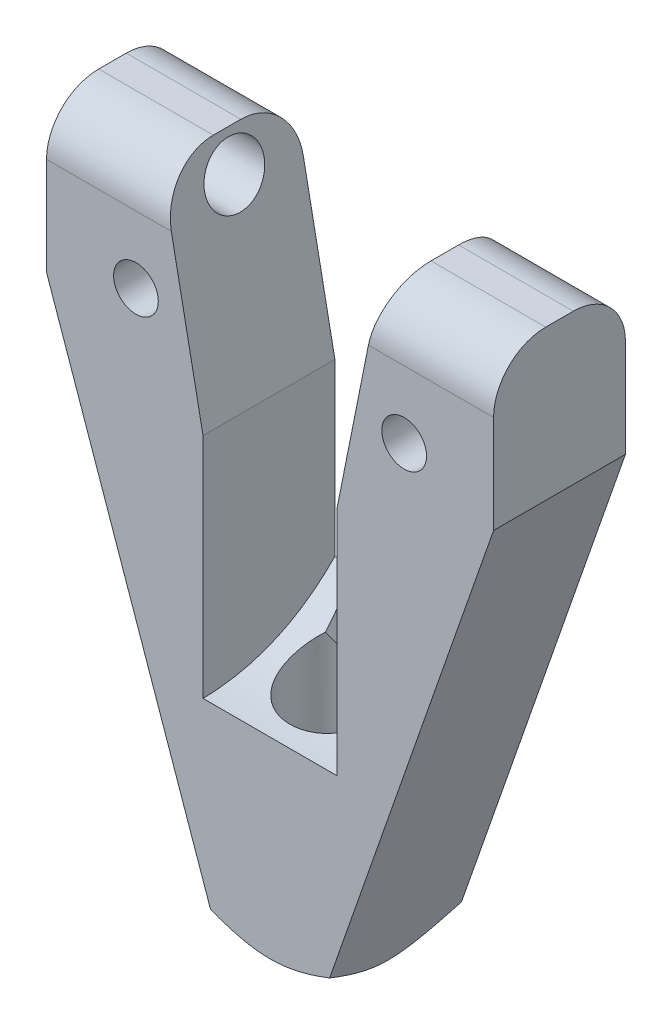
SolidWorks part; units mm, degrees
ref_plane "Front Plane" through (0, 0, 0) normal (0, 0, 1) x (1, 0, 0)
ref_plane "Top Plane" through (0, 0, 0) normal (0, 1, 0) x (1, 0, 0)
ref_plane "Right Plane" through (0, 0, 0) normal (1, 0, 0) x (0, 0, -1)
sketch "Sketch1" plane through (0, 0, 0) normal (0, 0, 1) x (1, 0, 0)
  line L22 (39, -51.5036) -> (34.8377, -51.5036)
  line L23 (39, -28) -> (39, -51.5036)
  line L24 (44.6, 0) -> (39, -28)
  line L25 (60, -20.1364) -> (60, 0)
  line L26 (60, -20.1364) -> (38.9512, -80.4124)
  line L27 (60, 0) -> (44.6, 0)
  line L28 (21.0488, -80.4124) -> (0, -20.1364)
  line L29 (0, -20.1364) -> (0, 0)
  line L30 (21, -51.5036) -> (21, -28.6)
  line L31 (25.1623, -51.5036) -> (21, -51.5036)
  line L32 (21, -28.6) -> (15.3764, 0)
  line L33 (0, 0) -> (15.3764, 0)
  line L34 (37, -86) -> (23, -86)
  line L35 (25.1623, -51.5036) -> (34.8377, -51.5036)
  circle A0 centre (48, -16) radius 3
  circle A1 centre (12, -16) radius 3
  spline S0 degree 3 poles (38.9512, -80.4124) (38.741, -81.0144) (38.5334, -81.6089) (38.3309, -82.1888) knots 0 0 0 0 0.25 0.25 0.25 0.25
  spline S1 degree 3 poles (38.3309, -82.1888) (38.1284, -82.7688) (37.9302, -83.3362) (37.7441, -83.869) knots 0.25 0.25 0.25 0.25 0.5 0.5 0.5 0.5
  spline S2 degree 3 poles (37.7441, -83.869) (37.6511, -84.1355) (37.5613, -84.3926) (37.4767, -84.6348) knots 0.5 0.5 0.5 0.5 0.625 0.625 0.625 0.625
  spline S3 degree 3 poles (37.4767, -84.6348) (37.3922, -84.877) (37.3127, -85.1045) (37.2423, -85.3061) knots 0.625 0.625 0.625 0.625 0.75 0.75 0.75 0.75
  spline S4 degree 3 poles (37.2423, -85.3061) (37.1719, -85.5076) (37.1112, -85.6816) (37.0682, -85.8048) knots 0.75 0.75 0.75 0.75 0.875 0.875 0.875 0.875
  spline S5 degree 2 poles (37.0682, -85.8048) (37.0252, -85.9279) (37, -86) knots 0.875 0.875 0.875 1 1 1
  spline S6 degree 2 poles (23, -86) (22.9755, -85.9299) (22.9325, -85.8066) knots 0 0 0 0.125 0.125 0.125
  spline S7 degree 3 poles (22.9325, -85.8066) (22.911, -85.745) (22.8847, -85.6697) (22.8553, -85.5855) knots 0.125 0.125 0.125 0.125 0.1875 0.1875 0.1875 0.1875
  spline S8 degree 3 poles (22.8553, -85.5855) (22.8258, -85.5013) (22.7932, -85.4079) (22.7583, -85.3078) knots 0.1875 0.1875 0.1875 0.1875 0.25 0.25 0.25 0.25
  spline S9 degree 3 poles (22.7583, -85.3078) (22.6883, -85.1074) (22.6089, -84.8801) (22.524, -84.637) knots 0.25 0.25 0.25 0.25 0.375 0.375 0.375 0.375
  spline S10 degree 3 poles (22.524, -84.637) (22.4392, -84.3939) (22.3487, -84.1348) (22.2555, -83.8681) knots 0.375 0.375 0.375 0.375 0.5 0.5 0.5 0.5
  spline S11 degree 3 poles (22.2555, -83.8681) (22.0692, -83.3346) (21.8716, -82.7687) (21.6691, -82.1889) knots 0.5 0.5 0.5 0.5 0.75 0.75 0.75 0.75
  spline S12 degree 3 poles (21.6691, -82.1889) (21.4667, -81.6091) (21.2591, -81.0146) (21.0488, -80.4124) knots 0.75 0.75 0.75 0.75 1 1 1 1
  dimension "D1" = 36
  dimension "D2" = 16
  dimension "D3" = 12
  dimension "D4" = 12
extrude "Boss-Extrude2" add sketch "Sketch1" along normal blind 17.7
ref_plane "Plane2" through (30, 0, 0) normal (-1, 0, 0) x (0, 0, 1)
sketch "Sketch2" plane through (30, 0, 0) normal (-1, 0, 0) x (0, 0, 1)
  line L0 (11.5, -86) -> (11.5, -81.75)
  line L1 (17.7, -86) -> (0, -86) construction
  line L2 (15.0441, -75) -> (15.0441, -57.48)
  line L3 (102, 6.2) -> (84.4804, 6.2)
  line L4 (113, 2.65) -> (108.7541, 2.65)
  line L5 (11.5, -86) -> (8.85, -86)
  line L6 (8.85, -86) -> (8.85, -57.48)
  line L7 (8.85, -57.48) -> (15.0441, -57.48)
  arc A0 (107.1067, 3.5159) -> (108.7541, 2.65) centre (108.7541, 4.65) ccw
  arc A1 (107.1067, 3.5159) -> (102, 6.2) centre (102, 0) ccw
  arc A2 (11.5, -81.75) -> (12.3644, -80.1037) centre (13.5, -81.75) cw
  arc A3 (12.3644, -80.1037) -> (15.0441, -75) centre (8.8441, -75) ccw
  point P8 (8.85, -86)
  dimension "D1" = 4.25
  dimension "D2" = 2
  dimension "D3" = 6.2
  dimension "D4" = 28.52
  dimension "D5" = 17.52
  dimension "D6" = 2.65
revolve "Cut-Revolve2" cut sketch "Sketch2" angle 360 about L6
sketch "Sketch3" plane through (30, 0, 0) normal (-1, 0, 0) x (0, 0, 1)
  line L0 (17.7, -20.1364) -> (17.7, -80.4124) construction
  line L2 (0, -51.5036) -> (17.7, -51.5036)
  line L3 (17.7, -51.5036) -> (17.7, -59.1523)
  line L4 (2.6559, -57.48) -> (15.0441, -57.48) construction
  spline S0 degree 2 poles (17.7, -59.1523) (7.3354, -59.0089) (0, -51.5036) knots 0 0 0 1 1 1
extrude "Cut-Extrude1" cut sketch "Sketch3" against normal up to surface and the other way up to surface up to face at (39, -39.7518, 8.85) other way up to face at (21, -40.0518, 8.85)
sketch "Sketch4" plane through (30, 0, 0) normal (-1, 0, 0) x (0, 0, 1)
  line L0 (4.1824, -56.4823) -> (-7.4784, -54.9866)
ref_plane "Plane4" through (0, 0, 8.85) normal (0, 0, -1) x (-1, 0, 0)
sketch "Sketch6" plane through (0, 0, 8.85) normal (0, 0, -1) x (-1, 0, 0)
  line L1 (-30, -56.4823) -> (-30, -54.9866) construction
  ellipse E0 centre (-30, -47.9683) end of major axis (-30, -35.7103) minor radius 6.4919
extrude "Cut-Extrude2" cut sketch "Sketch6" along normal blind 48.7
sketch "Sketch7" plane through (0, 0, 0) normal (0, 1, 0) x (1, 0, 0)
  circle A0 centre (30, -8.85) radius 6.1941
extrude "Cut-Extrude3" cut sketch "Sketch7" against normal blind 60.7
ref_plane "Plane5" through (6, 0, 0) normal (-1, 0, 0) x (0, 0, 1)
sketch "Sketch8" plane through (6, 0, 0) normal (-1, 0, 0) x (0, 0, 1)
  line L0 (17.7, 0) -> (0, 0) construction
  line L1 (17.7, -86) -> (0, -86) construction
  circle A0 centre (8.85, -5) radius 4
  point P7 (8.85, -86)
  dimension "D1" = 8
  dimension "D2" = 5
extrude "Cut-Extrude4" cut sketch "Sketch8" against normal blind 48
fillet "Fillet1" radius 7 4 edges at (52.3, 0, 17.7) (52.3, 0, 0) (7.6882, 0, 0) (7.6882, 0, 17.7)
sketch "Sketch10" plane through (0, -86, 0) normal (0, -1, 0) x (1, 0, 0)
  circle A0 centre (30, 8.85) radius 7
  dimension "D1" = 14
extrude "Cut-Extrude5" cut sketch "Sketch10" against normal blind 48 draft 60 flip side to cut
ref_plane "Plane6" through (0, -5, 0) normal (0, 1, 0) x (1, 0, 0)
